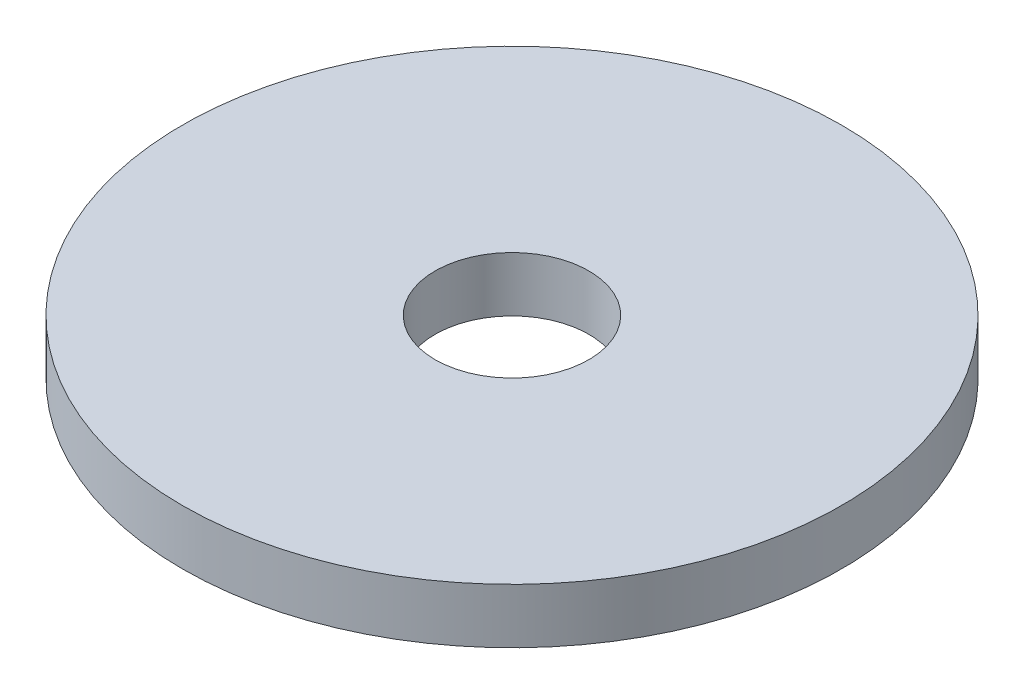
from build123d import *

# Parameters (mm, degrees)
SKETCH_1_R          = 30
SKETCH_1_R_2        = 7
BOSS_EXTRUDE1_DEPTH = 5


with BuildPart() as part:
    # Sketch 1 → Boss-Extrude1 (new body)
    with BuildSketch(Plane(origin=(0, 0, 0), x_dir=(1, 0, 0), z_dir=(0, 1, 0))):
        with Locations(Location((0, 0, 0), (0, 0, 270))):
            Circle(SKETCH_1_R)
        with Locations(Location((0, 0, 0), (0, 0, 270))):
            Circle(SKETCH_1_R_2, mode=Mode.SUBTRACT)
    extrude(amount=BOSS_EXTRUDE1_DEPTH)


solid = part.part
